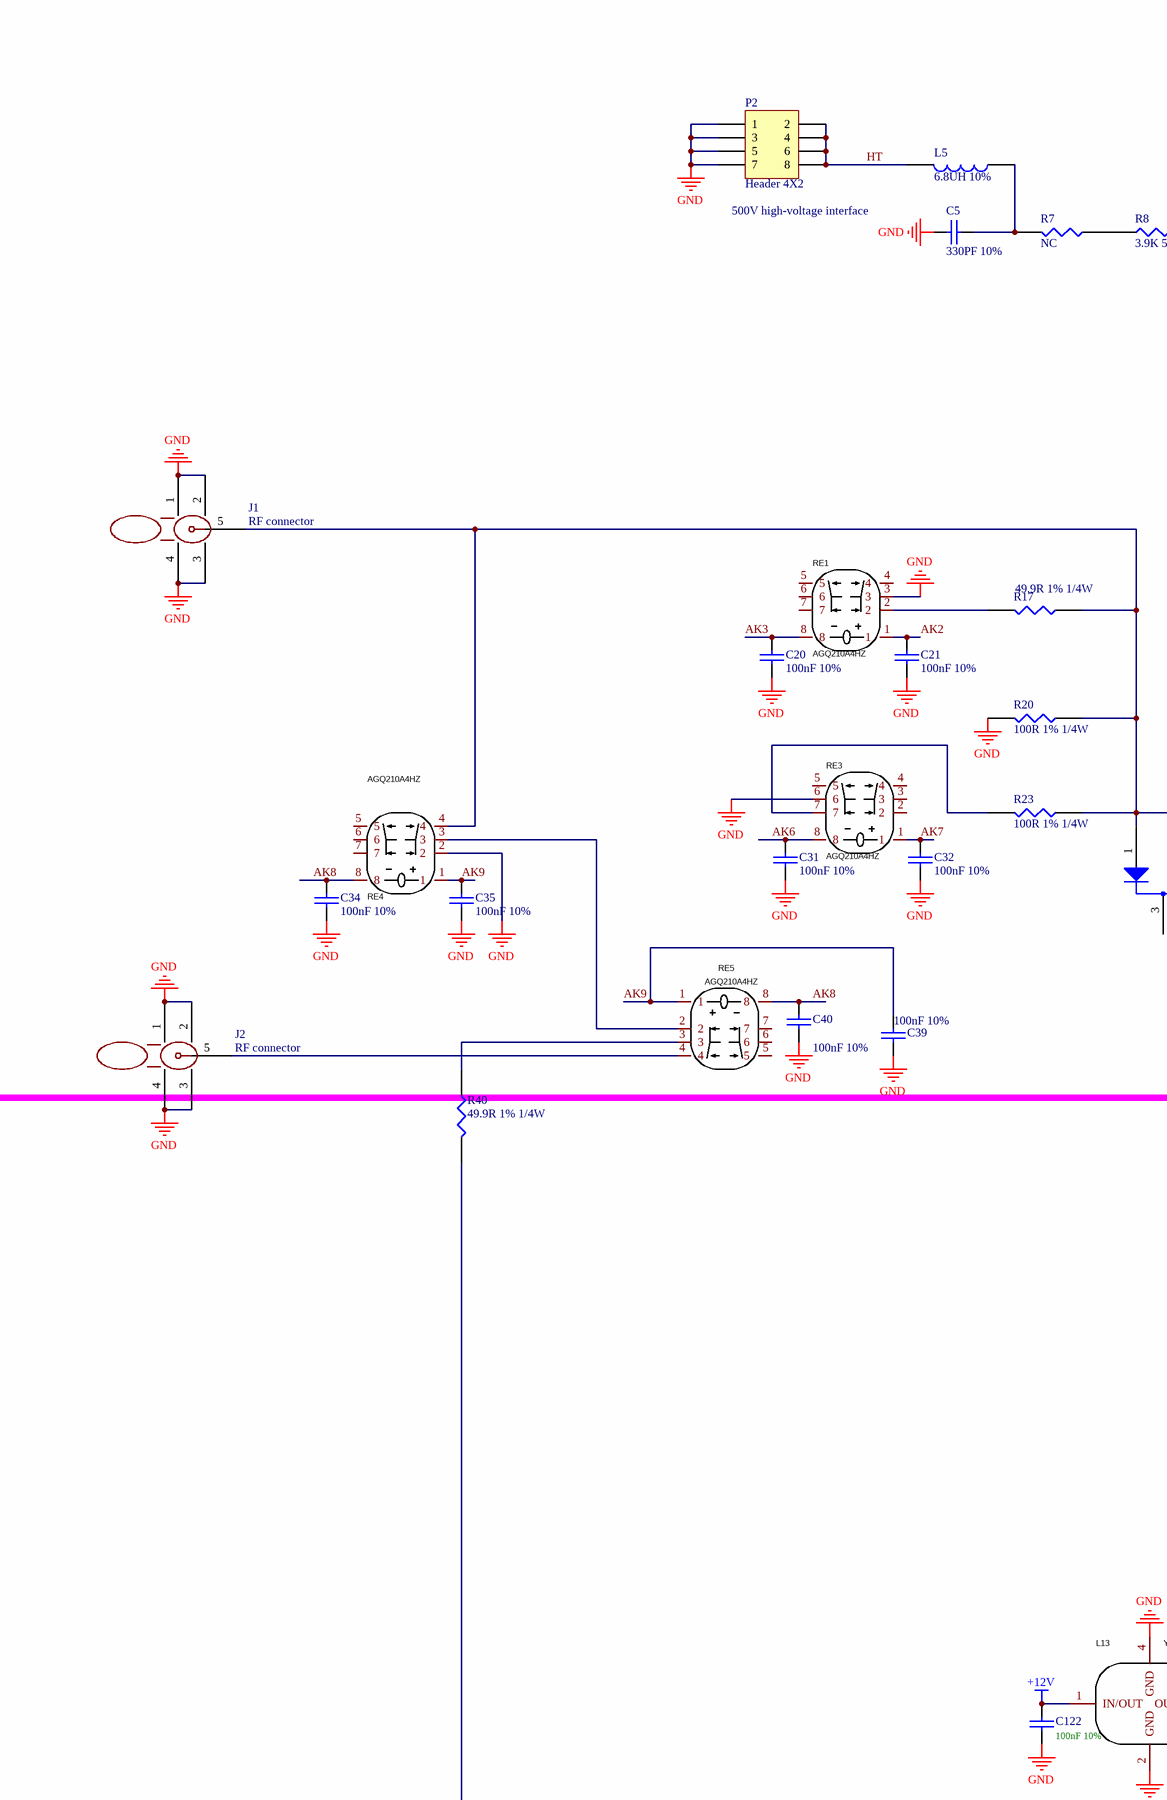
[diagram p0: PCBE109560-7.SchDoc, top left]
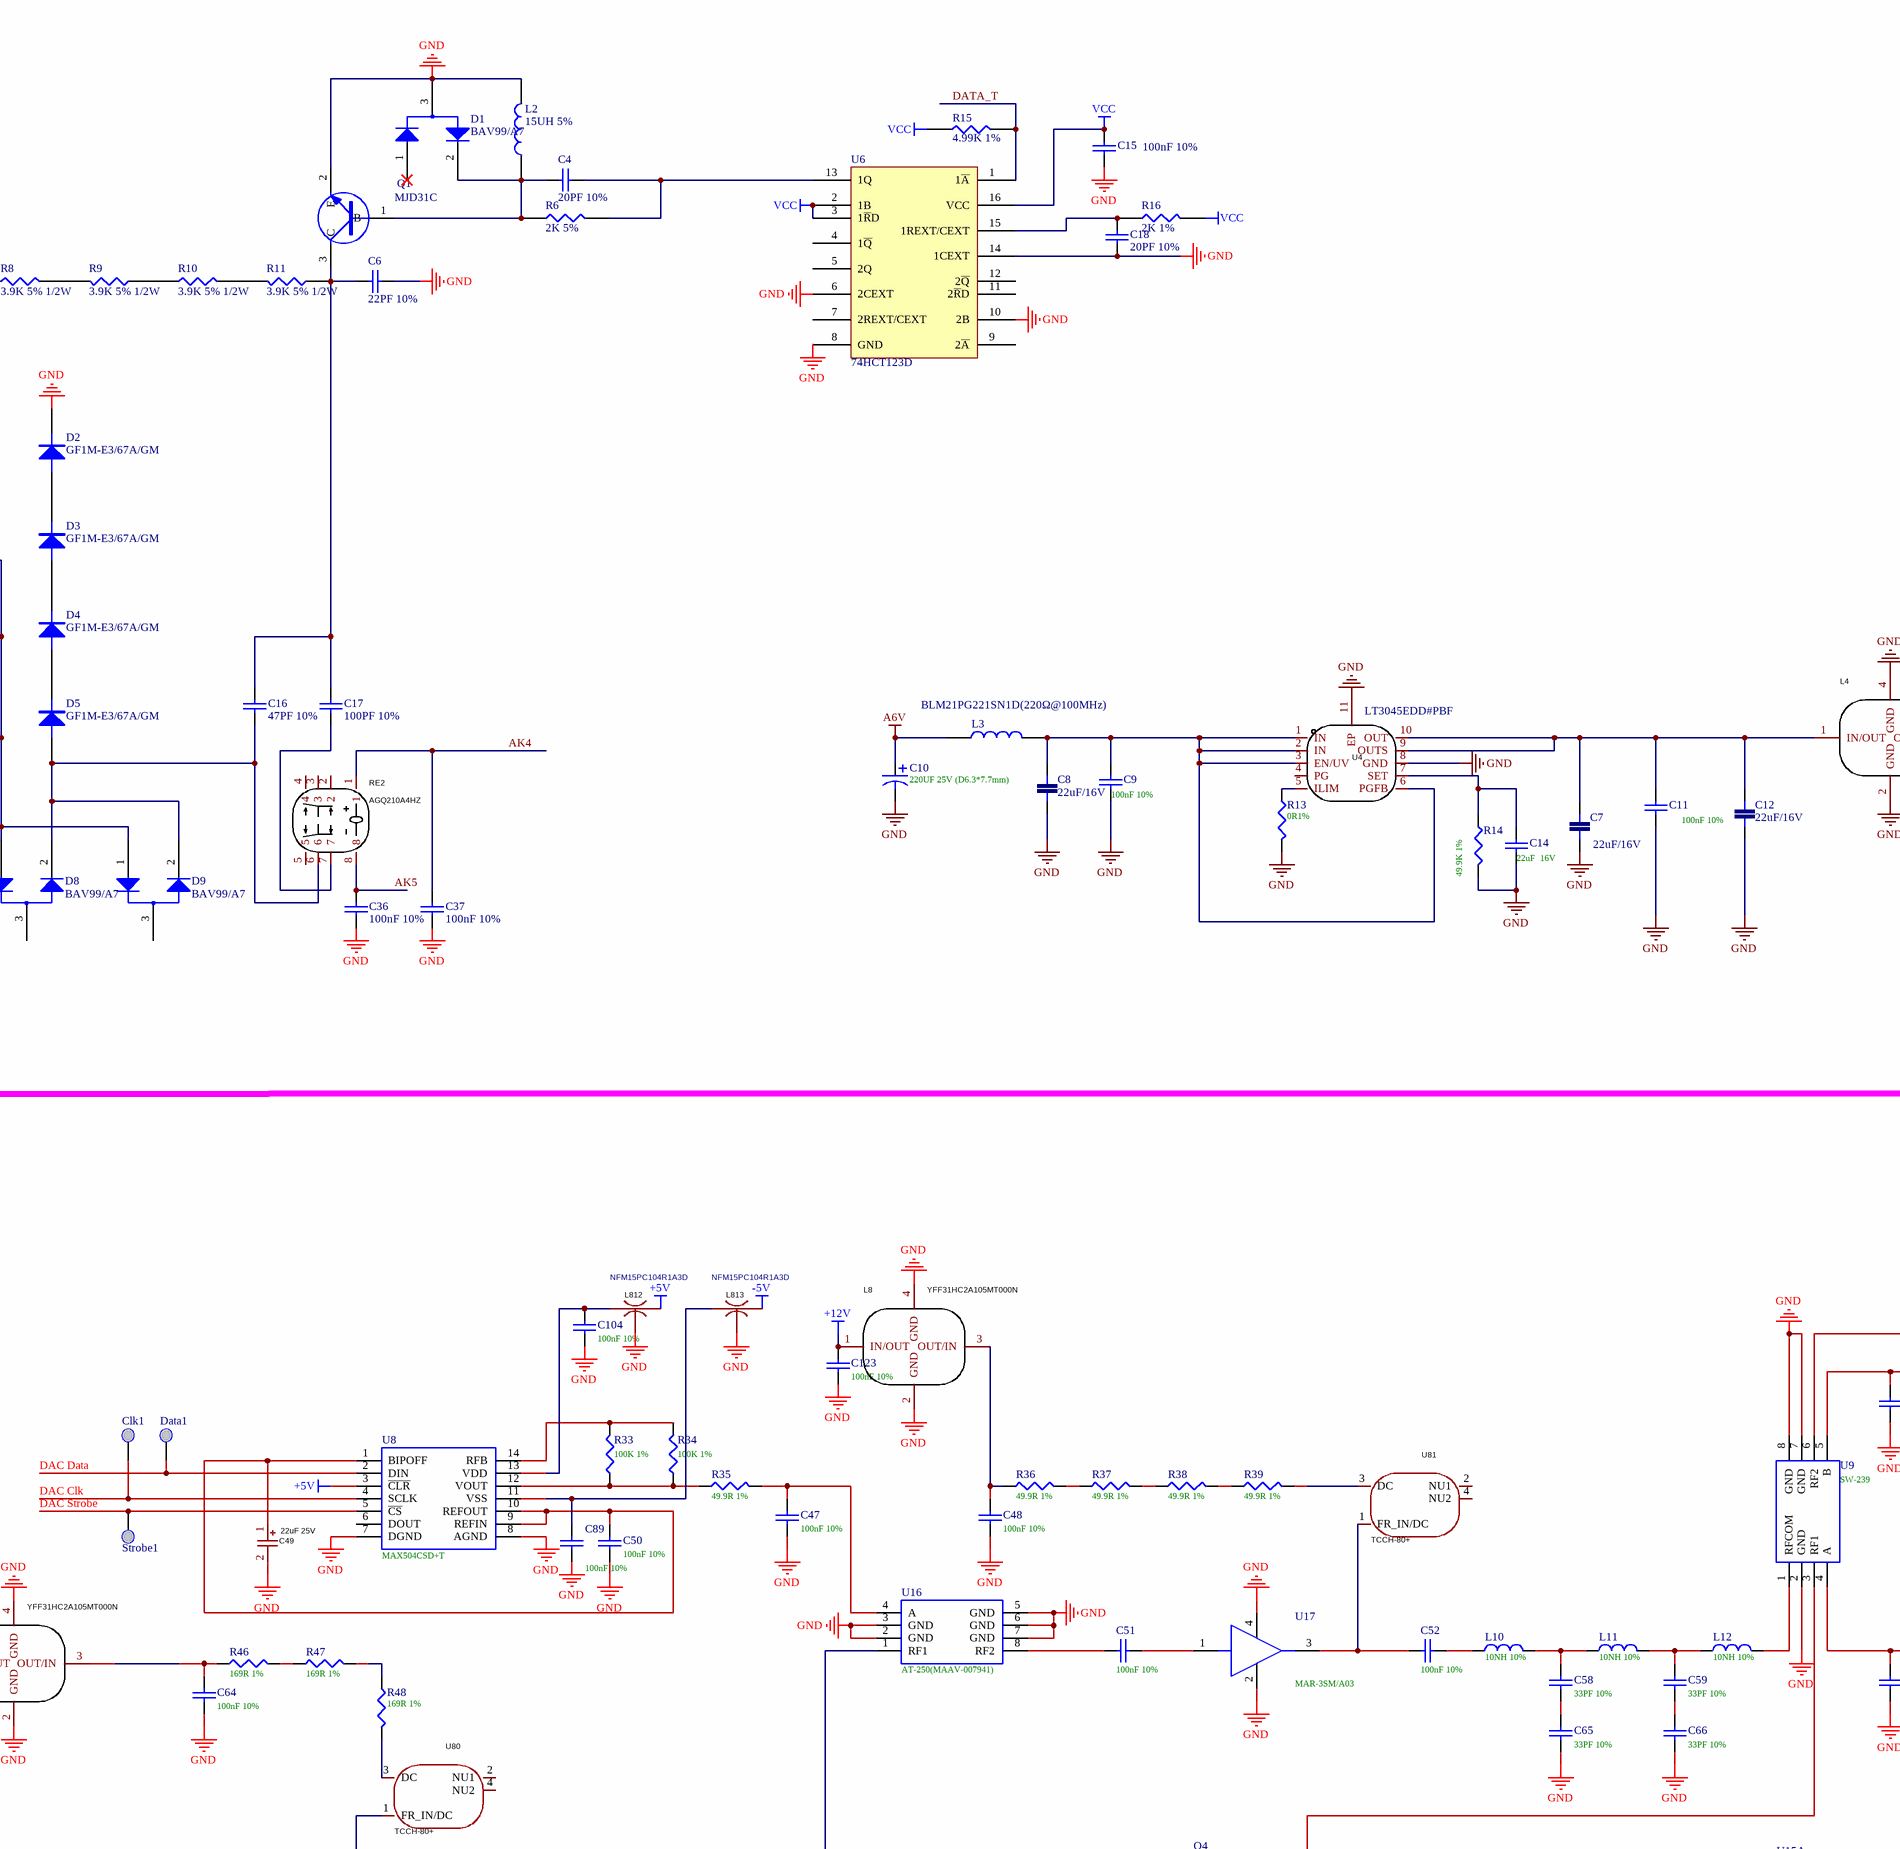
[diagram p1: PCBE109560-7.SchDoc, top middle]
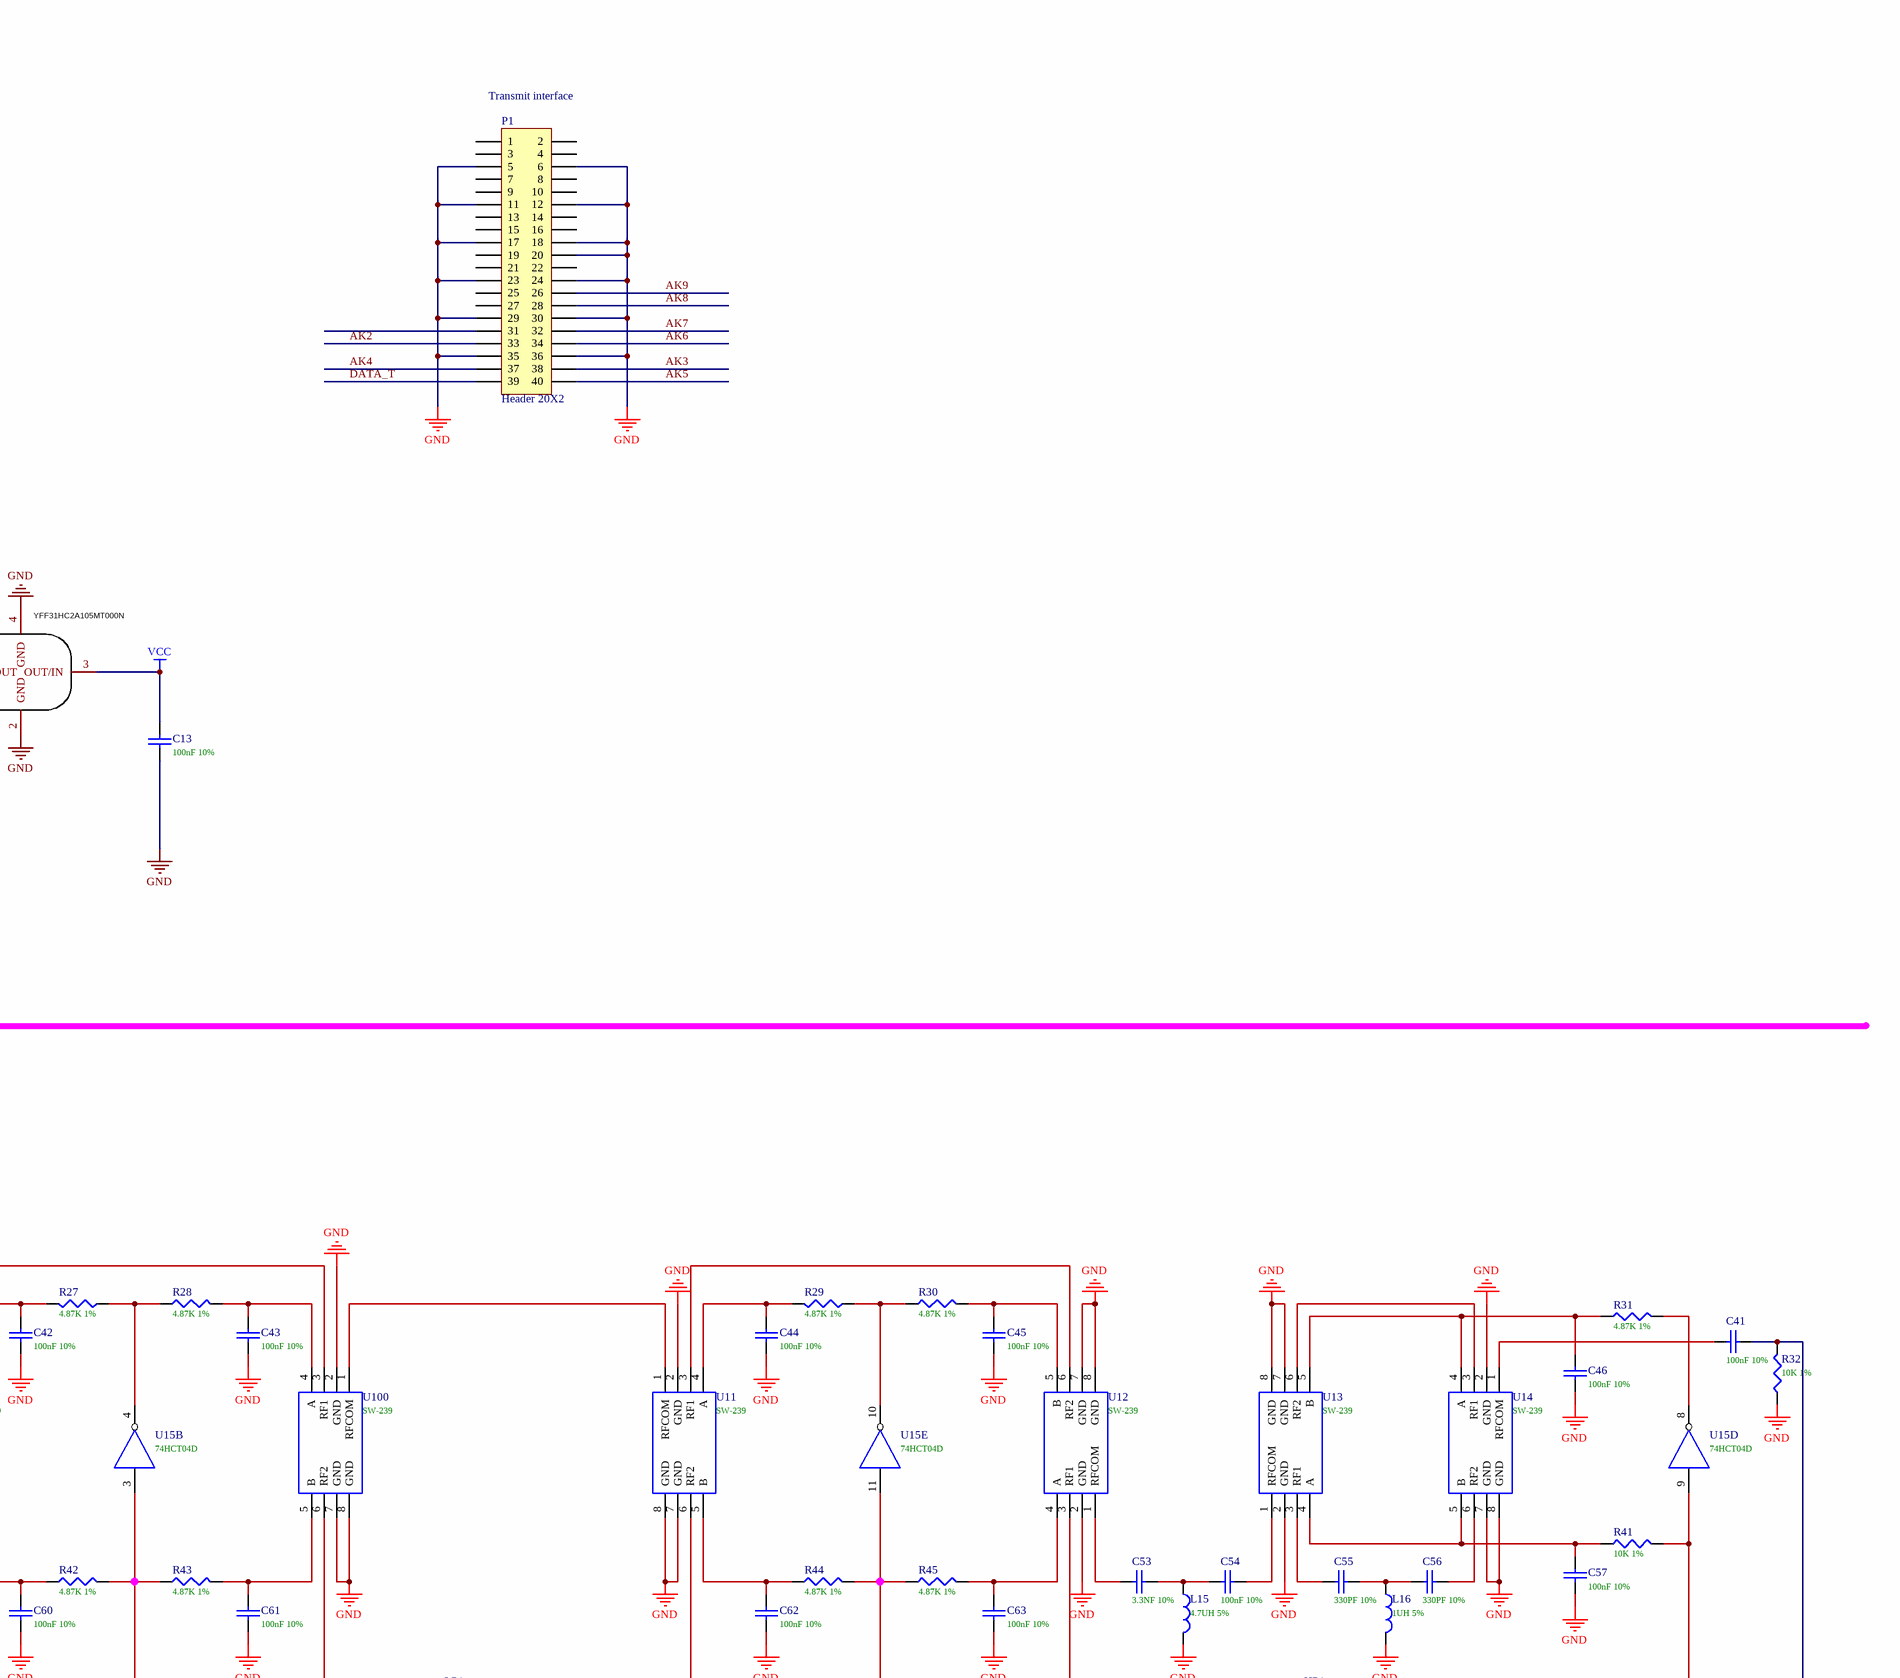
[diagram p2: PCBE109560-7.SchDoc, top right]
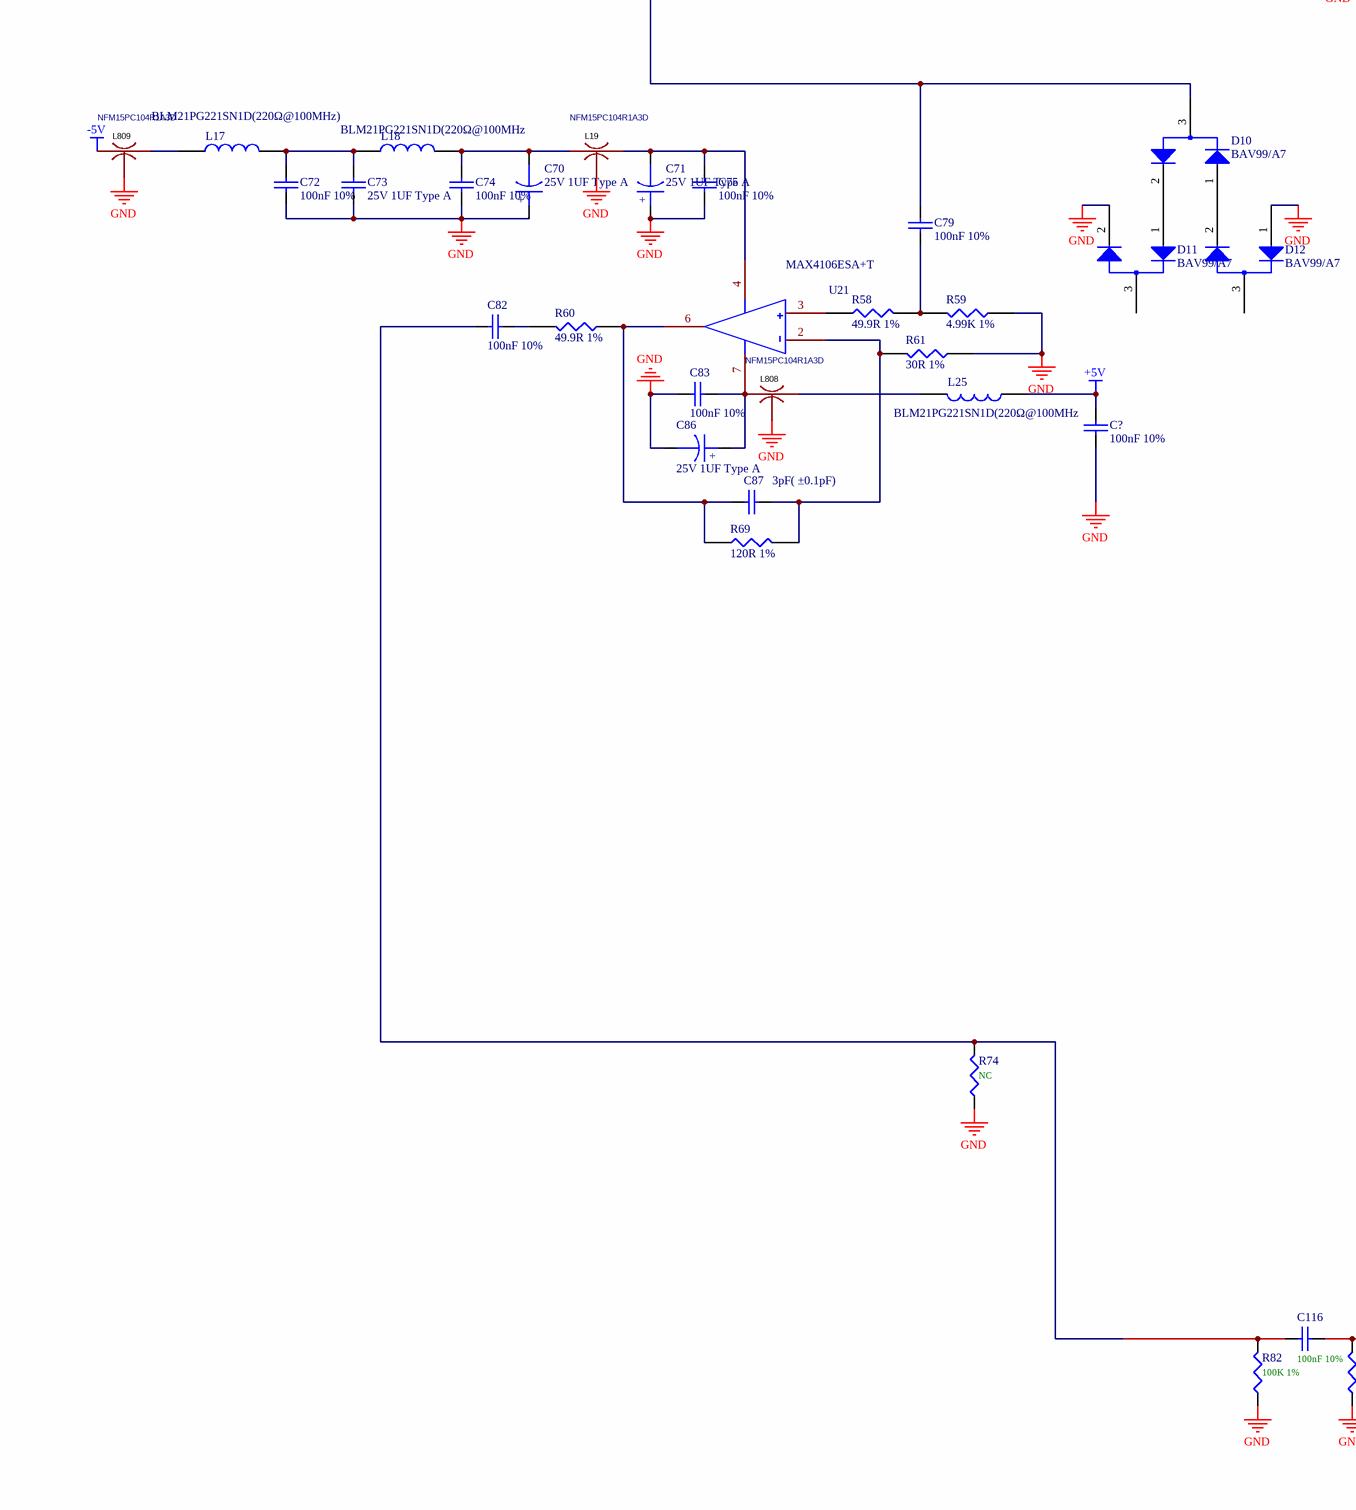
[diagram p3: PCBE109560-7.SchDoc, bottom left]
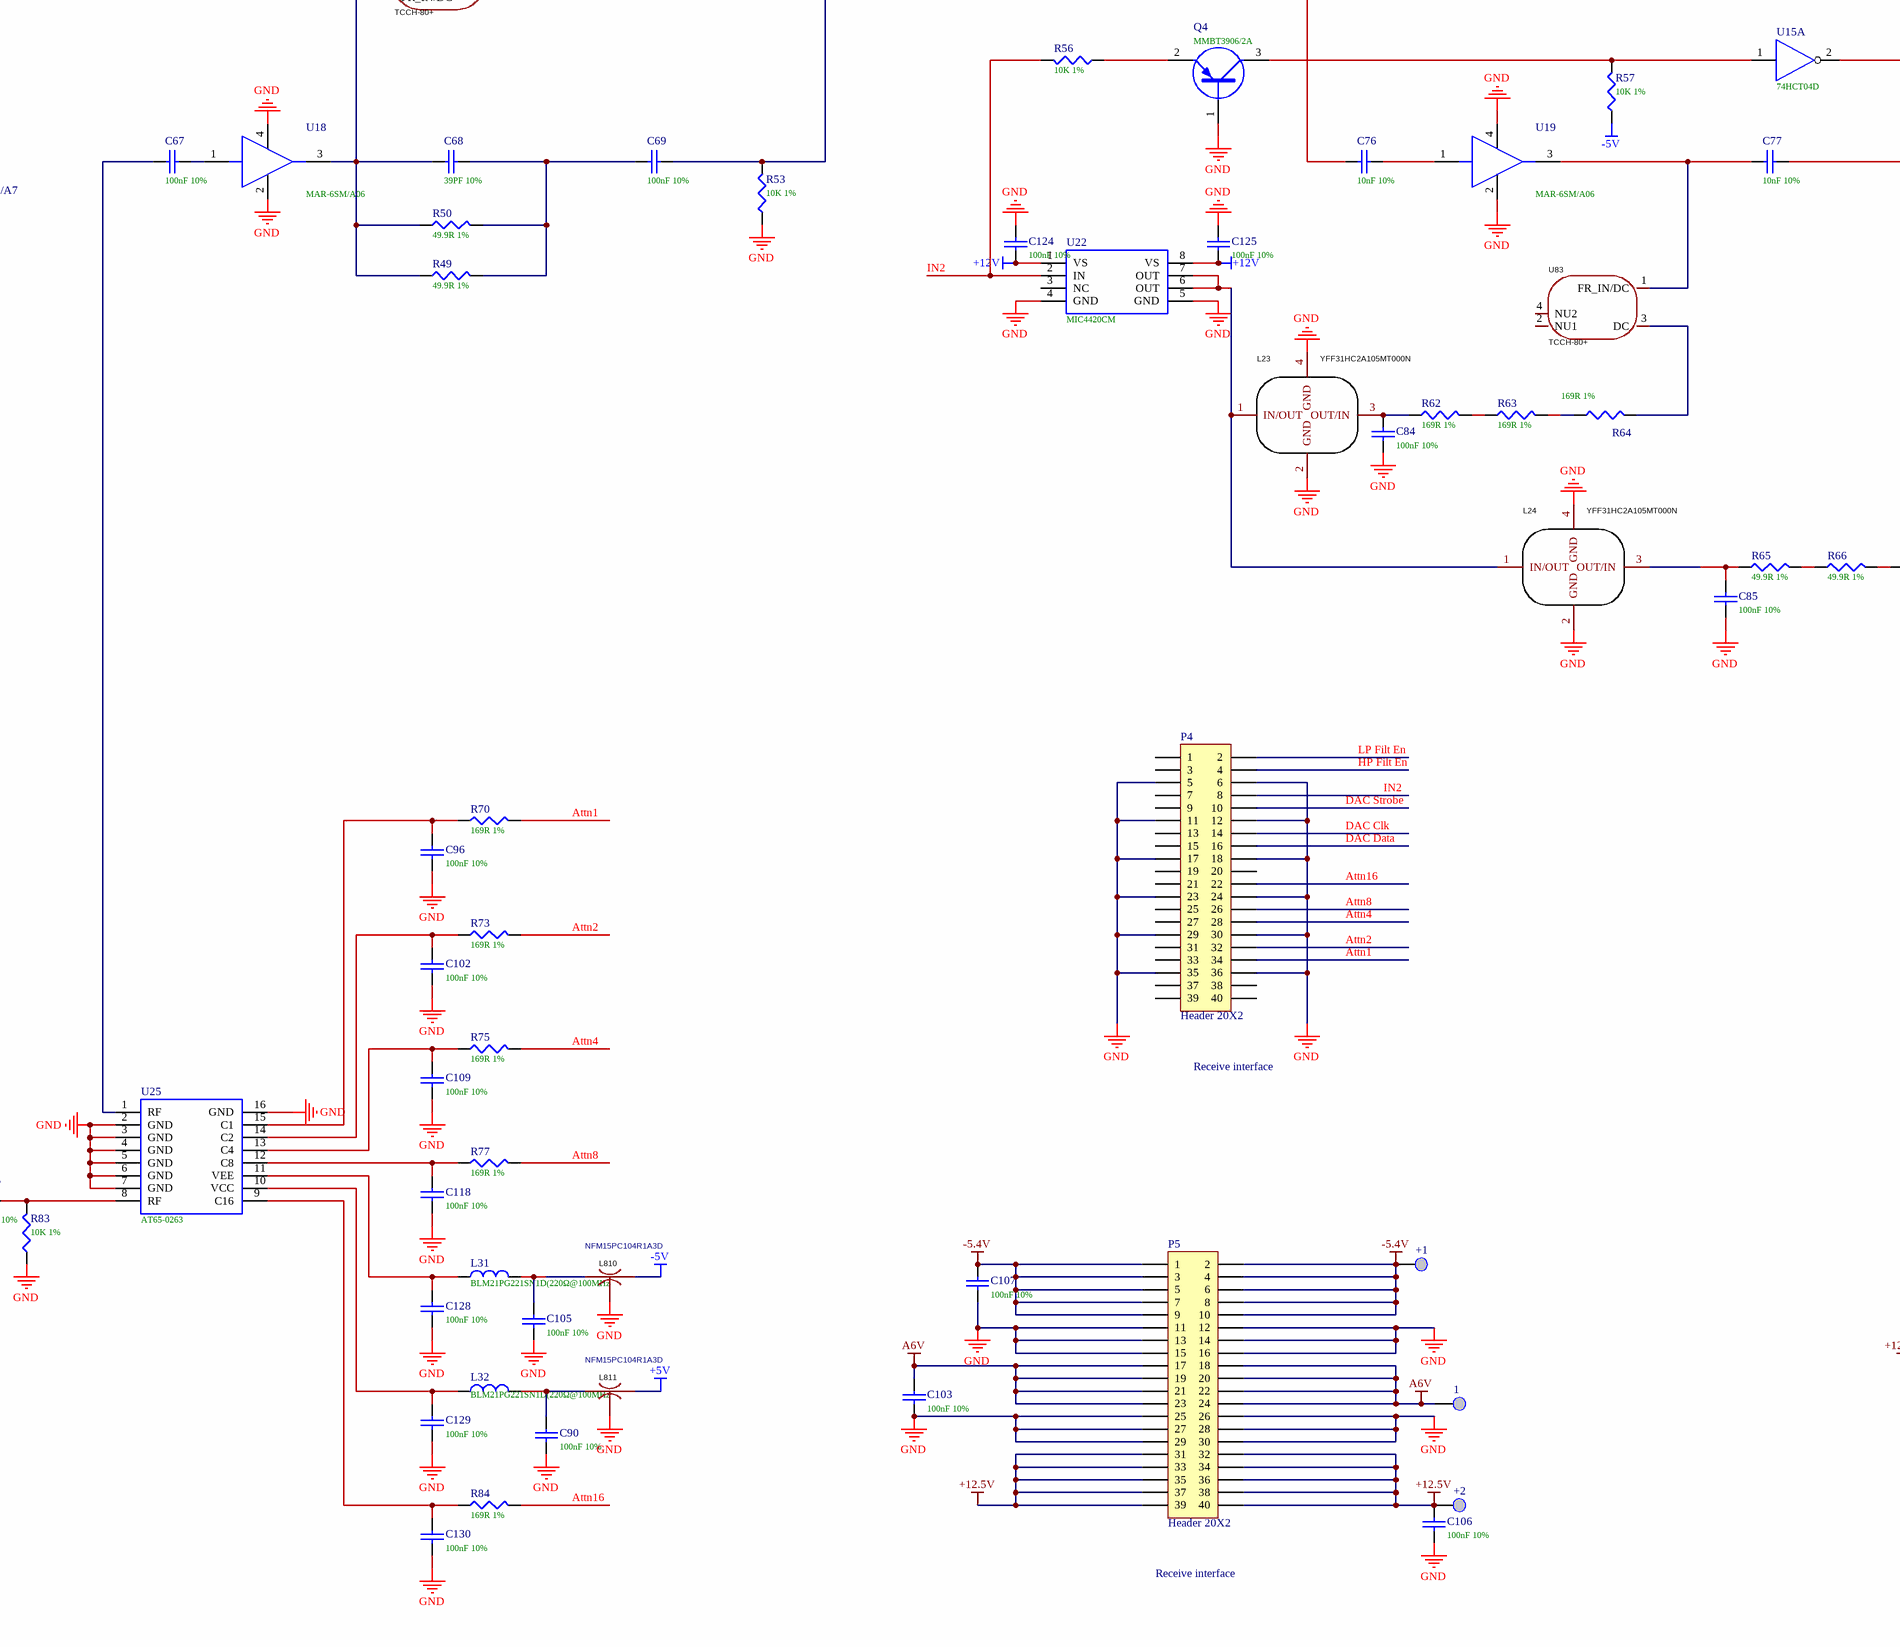
[diagram p4: PCBE109560-7.SchDoc, bottom middle]
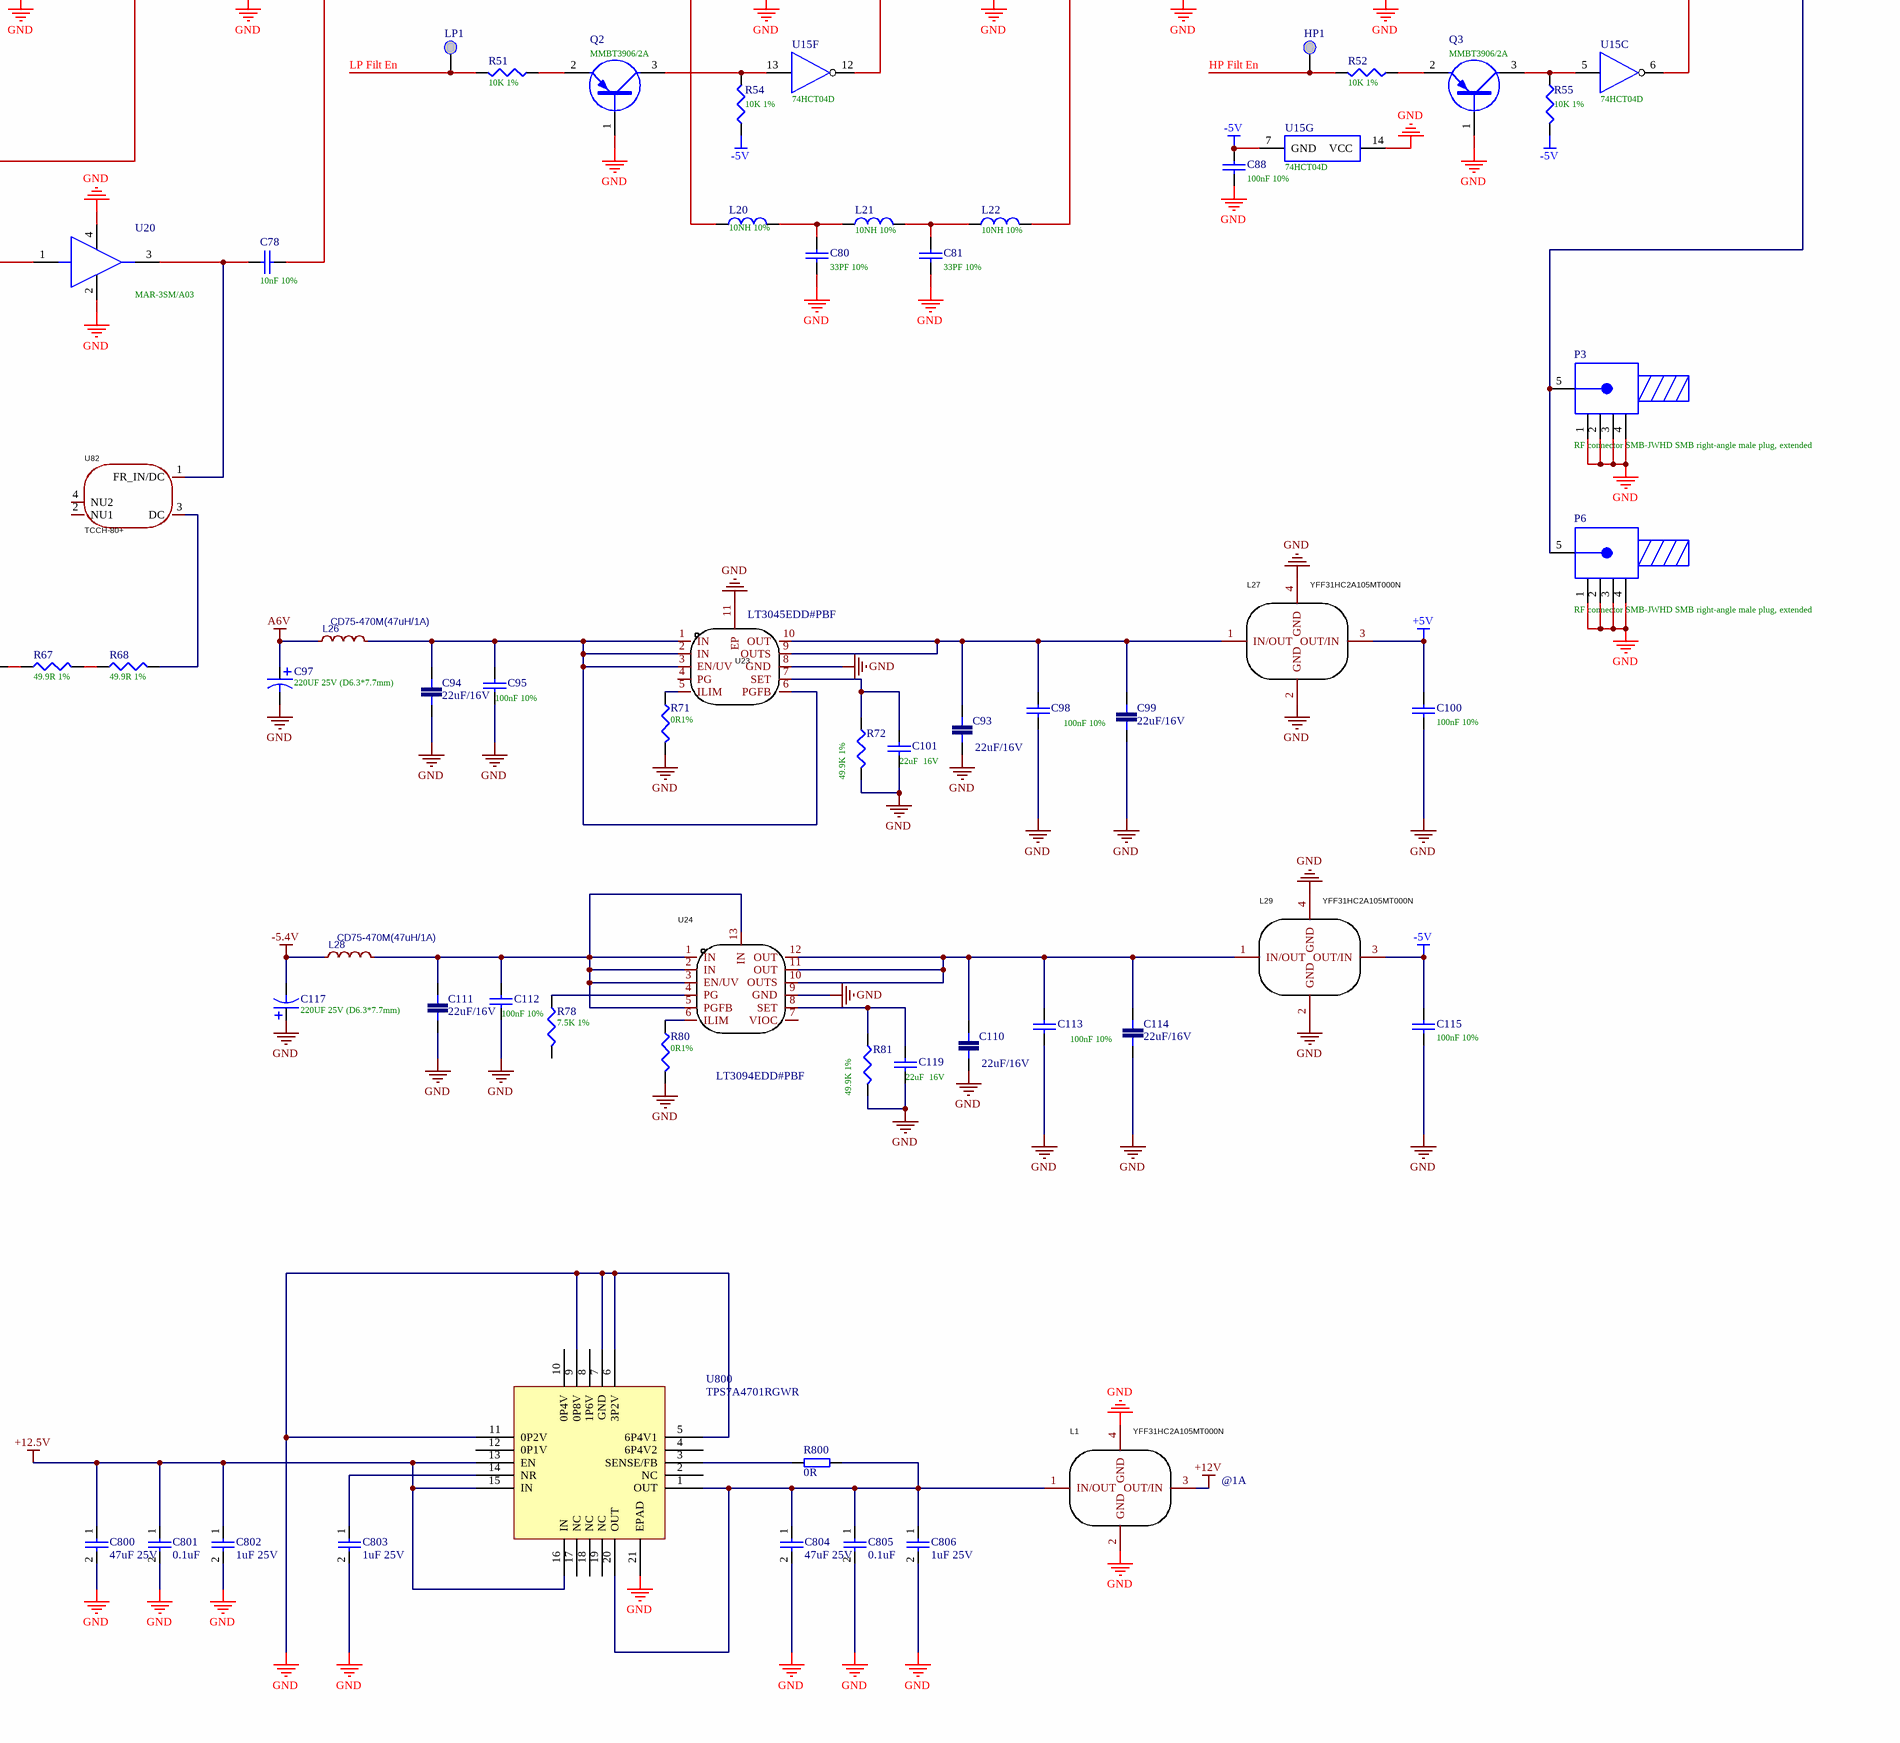
[diagram p5: PCBE109560-7.SchDoc, bottom right]
# Altium schematic sheet PCBE109560-7.SchDoc (part 1 of 2)
size E; SheetNumber: 0; SheetTotal: 0